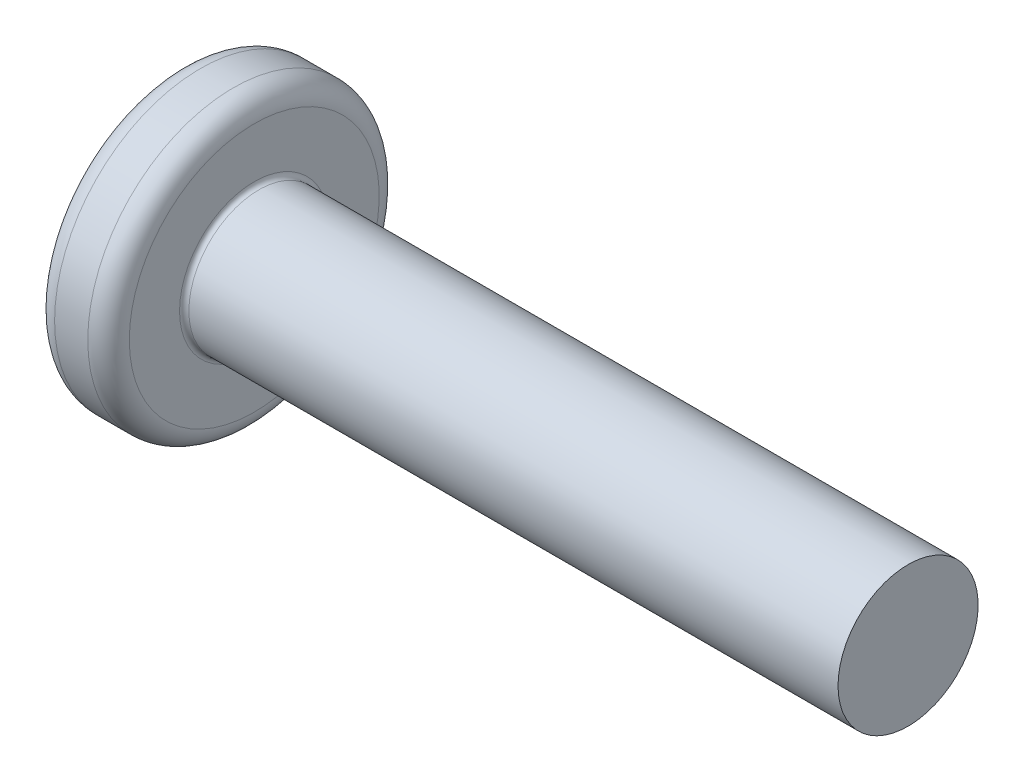
from build123d import *


with BuildPart() as part:
    # Dimensioned Sketch → Revolve3 (revolve)
    with BuildSketch(Plane.XY, mode=Mode.PRIVATE) as revolve3_sk:
        with BuildLine():
            Line((0, 0), (0, 2.6752))
            ThreePointArc((0, 2.6752), (0.130278904, 2.989721096), (0.4448, 3.12))
            Line((0.4448, 3.12), (1.1552, 3.12))
            ThreePointArc((1.1552, 3.12), (1.469721096, 2.989721096), (1.6, 2.6752))
            Line((1.6, 2.6752), (1.6, 1.6))
            ThreePointArc((1.6, 1.6), (1.629289322, 1.529289322), (1.7, 1.5))
            Line((1.7, 1.5), (15.6, 1.5))
            Line((15.6, 1.5), (15.6, 0))
            Line((15.6, 0), (0, 0))
        make_face()
    revolve(revolve3_sk.sketch.rotate(Axis((0, 0, 0), (1, 0, 0)), 90), axis=Axis((0, 0, 0), (1, 0, 0)))


solid = part.part
